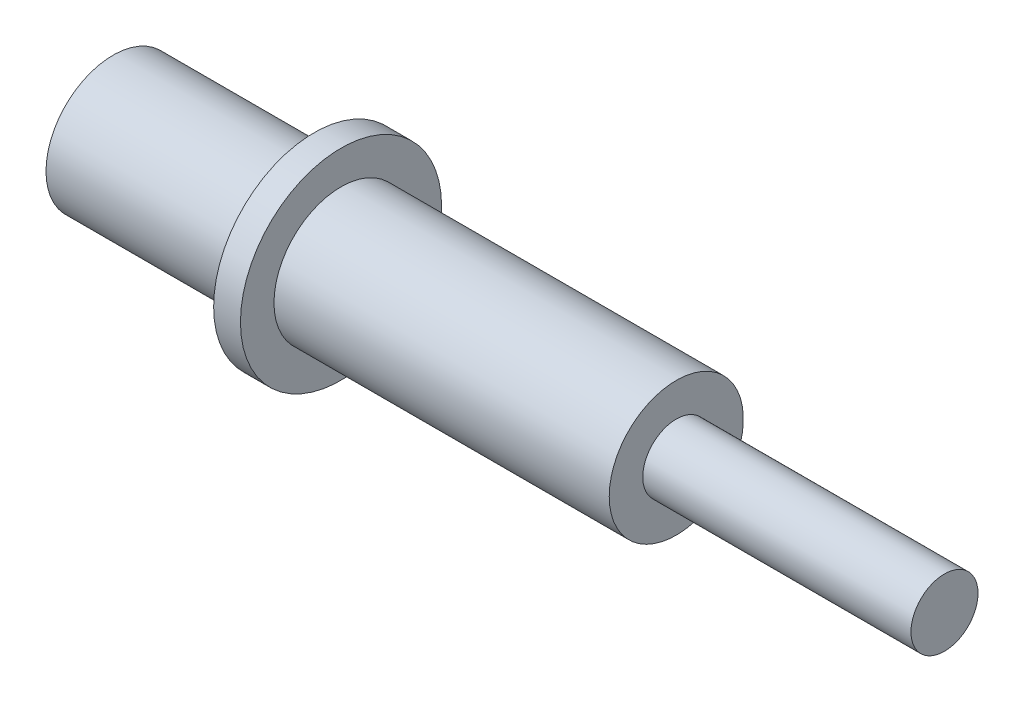
SolidWorks part; units mm, degrees
ref_plane "前视基准面" through (0, 0, 0) normal (0, 0, 1) x (1, 0, 0)
ref_plane "上视基准面" through (0, 0, 0) normal (0, 1, 0) x (1, 0, 0)
ref_plane "右视基准面" through (0, 0, 0) normal (1, 0, 0) x (0, 0, -1)
sketch "草图1" plane through (0, 0, 0) normal (1, 0, 0) x (0, 0, -1)
  circle A0 centre (0, 0) radius 2.5
  dimension "D1" = 5
extrude "凸台-拉伸1" add sketch "草图1" along normal blind 20
sketch "草图2" plane through (0, 0, 0) normal (-1, 0, 0) x (0, 0, 1)
  circle A0 centre (0, 0) radius 5
  dimension "D1" = 10
extrude "凸台-拉伸2" add sketch "草图2" along normal blind 25
sketch "草图3" plane through (-25, 0, 0) normal (-1, 0, 0) x (0, 0, 1)
  circle A0 centre (0, 0) radius 7.5
  dimension "D1" = 15
extrude "凸台-拉伸3" add sketch "草图3" along normal blind 2
sketch "草图4" plane through (-27, 0, 0) normal (-1, 0, 0) x (0, 0, 1)
  circle A0 centre (0, 0) radius 5
  dimension "D1" = 10
extrude "凸台-拉伸4" add sketch "草图4" along normal blind 15
